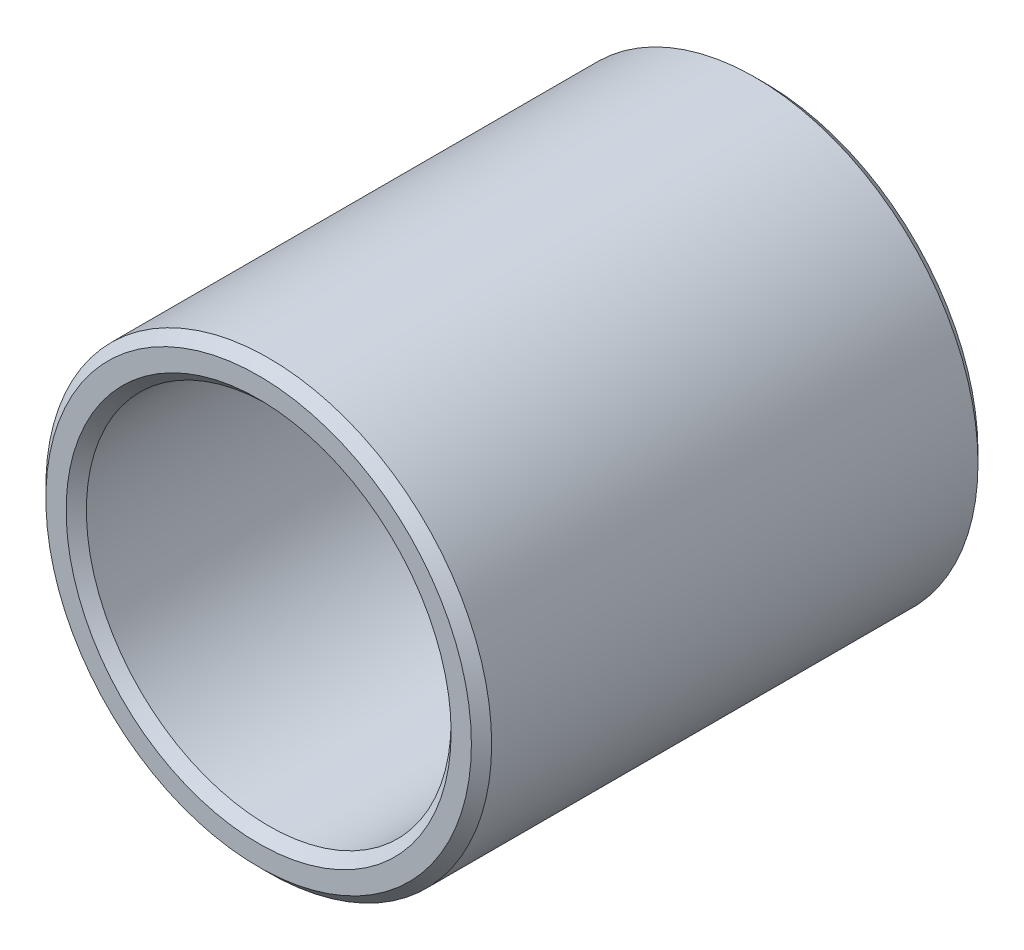
SolidWorks part; units mm, degrees
ref_plane "前视基准面" through (0, 0, 0) normal (0, 0, 1) x (1, 0, 0)
ref_plane "上视基准面" through (0, 0, 0) normal (0, 1, 0) x (1, 0, 0)
ref_plane "右视基准面" through (0, 0, 0) normal (1, 0, 0) x (0, 0, -1)
sketch "草图1" plane through (0, 0, 0) normal (0, 0, 1) x (1, 0, 0)
  circle A0 centre (0, 0) radius 11
  circle A1 centre (0, 0) radius 9
  dimension "D1" = 22
  dimension "D2" = 18
extrude "凸台-拉伸1" add sketch "草图1" along normal blind 25
chamfer "倒角1" distance 0.5 angle 45 4 edges at (9, 0, 25) (11, 0, 25) (9, 0, 0) (11, 0, 0)
